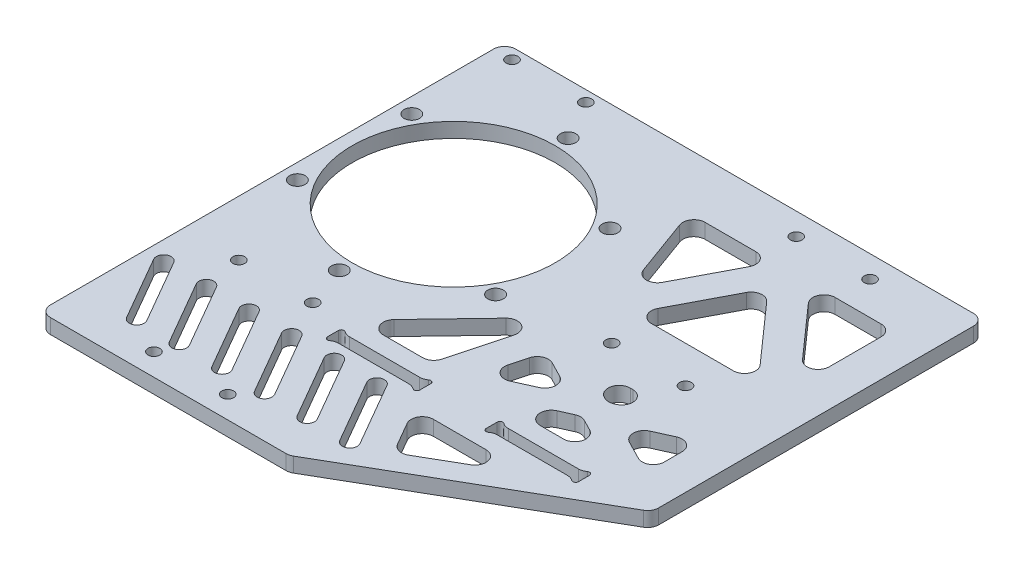
from build123d import *

# Parameters (mm, degrees)
SKETCH_1_W          = 130
SKETCH_1_H          = 90
SKETCH_1_R          = 27.5
SKETCH_1_R_2        = 2.1
SKETCH_1_R_3        = 1.6
EXTRUDE_1_DEPTH     = 4
EXTRUDE_2_DEPTH     = 4
SKETCH_3_R          = 1.6
CUT_EXTRUDE_1_DEPTH = 10
SKETCH_4_R          = 1.6
CUT_EXTRUDE_2_DEPTH = 10
CUT_EXTRUDE_3_DEPTH = 10
FILLET_1_R          = 3
CUT_EXTRUDE_4_DEPTH = 10
FILLET_2_R          = 3


with BuildPart() as part:
    # 草图1 → 凸台-拉伸1 (new body)
    with BuildSketch(Plane(origin=(0, 0, 0), x_dir=(1, 0, 0), z_dir=(0, 1, 0))):
        with Locations((65, 45)):
            Rectangle(SKETCH_1_W, SKETCH_1_H)
        with Locations(Location((31, 45.2, 0), (0, 0, 270))):
            Circle(SKETCH_1_R, mode=Mode.SUBTRACT)
        with Locations(Location((31, 76.2, 0), (0, 0, 270))):
            Circle(SKETCH_1_R_2, mode=Mode.SUBTRACT)
        with Locations(Location((57.846787517, 60.7, 0), (0, 0, 270))):
            Circle(SKETCH_1_R_2, mode=Mode.SUBTRACT)
        with Locations(Location((57.846787517, 29.7, 0), (0, 0, 270))):
            Circle(SKETCH_1_R_2, mode=Mode.SUBTRACT)
        with Locations(Location((31, 14.2, 0), (0, 0, 270))):
            Circle(SKETCH_1_R_2, mode=Mode.SUBTRACT)
        with Locations(Location((4.153212483, 29.7, 0), (0, 0, 270))):
            Circle(SKETCH_1_R_2, mode=Mode.SUBTRACT)
        with Locations(Location((4.153212483, 60.7, 0), (0, 0, 270))):
            Circle(SKETCH_1_R_2, mode=Mode.SUBTRACT)
        with Locations(Location((15, 3, 0), (0, 0, 270))):
            Circle(SKETCH_1_R_3, mode=Mode.SUBTRACT)
        with Locations(Location((35, 3, 0), (0, 0, 270))):
            Circle(SKETCH_1_R_3, mode=Mode.SUBTRACT)
    extrude(amount=EXTRUDE_1_DEPTH)

    # 草图2 → 凸台-拉伸2 (add)
    with BuildSketch(Plane(origin=(0, 4, 0), x_dir=(1, 0, 0), z_dir=(0, 1, 0))):
        Polygon((130, 0), (67.646170928, -36), (0, -36), (0, 0), align=None)
    extrude(amount=-EXTRUDE_2_DEPTH)

    # 草图3 → 切除-拉伸1 (cut)
    with BuildSketch(Plane(origin=(0, 4, 0), x_dir=(1, 0, 0), z_dir=(0, 1, 0))):
        with Locations(Location((25, -30, 0), (0, 0, 270))):
            Circle(SKETCH_3_R)
        with Locations(Location((45, -30, 0), (0, 0, 270))):
            Circle(SKETCH_3_R)
    extrude(amount=-CUT_EXTRUDE_1_DEPTH, mode=Mode.SUBTRACT)

    # 草图4 → 切除-拉伸2 (cut)
    with BuildSketch(Plane(origin=(0, 4, 0), x_dir=(1, 0, 0), z_dir=(0, 1, 0))):
        with Locations(Location((85, 84, 0), (0, 0, 270))):
            Circle(SKETCH_4_R)
        with Locations(Location((105, 84, 0), (0, 0, 270))):
            Circle(SKETCH_4_R)
        with Locations(Location((85, 34, 0), (0, 0, 270))):
            Circle(SKETCH_4_R)
        with Locations(Location((105, 34, 0), (0, 0, 270))):
            Circle(SKETCH_4_R)
        with Locations(Location((5, 87, 0), (0, 0, 270))):
            Circle(SKETCH_4_R)
        with Locations(Location((25, 87, 0), (0, 0, 270))):
            Circle(SKETCH_4_R)
    extrude(amount=-CUT_EXTRUDE_2_DEPTH, mode=Mode.SUBTRACT)

    # 草图2<3> → 切除-拉伸3 (cut)
    with BuildSketch(Plane(origin=(0, 4, 0), x_dir=(1, 0, 0), z_dir=(0, 1, 0))):
        with BuildLine():
            Line((46.5, 0), (45, 0))
            Line((45, 0), (45, -3))
            ThreePointArc((45, -3), (45.75, -3.75), (46.5, -3))
            Line((46.5, -3), (68.5, -3))
            ThreePointArc((68.5, -3), (69.25, -3.75), (70, -3))
            Line((70, -3), (70, 0))
            Line((70, 0), (68.5, 0))
            Line((68.5, 0), (46.5, 0))
        make_face()
        with BuildLine():
            Line((113, -3), (113, 0))
            Line((113, 0), (111.5, 0))
            Line((111.5, 0), (89.5, 0))
            Line((89.5, 0), (88, 0))
            Line((88, 0), (88, -3))
            ThreePointArc((88, -3), (88.75, -3.75), (89.5, -3))
            Line((89.5, -3), (111.5, -3))
            ThreePointArc((111.5, -3), (112.25, -3.75), (113, -3))
        make_face()
        with BuildLine():
            ThreePointArc((46.5, 0), (45.75, 0.75), (45, 0))
            Line((45, 0), (46.5, 0))
        make_face()
        with BuildLine():
            Line((68.5, 0), (70, 0))
            ThreePointArc((70, 0), (69.25, 0.75), (68.5, 0))
        make_face()
        with BuildLine():
            Line((88, 0), (89.5, 0))
            ThreePointArc((89.5, 0), (88.75, 0.75), (88, 0))
        make_face()
        with BuildLine():
            Line((111.5, 0), (113, 0))
            ThreePointArc((113, 0), (112.25, 0.75), (111.5, 0))
        make_face()
    extrude(amount=-CUT_EXTRUDE_3_DEPTH, mode=Mode.SUBTRACT)

    # 圆角1
    fillet_1_edges = [part.edges().sort_by_distance(p)[0] for p in [
        (67.646170928, 2, 36),
        (0, 2, 36),
        (0, 2, -90),
        (130, 2, -90),
        (130, 2, 0),
    ]]
    fillet(fillet_1_edges, radius=FILLET_1_R)

    # 草图5 → 切除-拉伸4 (cut)
    with BuildSketch(Plane(origin=(0, 4, 0), x_dir=(1, 0, 0), z_dir=(0, 1, 0))):
        with BuildLine():
            Line((6.732050808, -6.339745962), (16.732050808, -23.660254038))
            ThreePointArc((16.732050808, -23.660254038), (16, -26.392304845), (13.267949192, -25.660254038))
            Line((13.267949192, -25.660254038), (3.267949192, -8.339745962))
            ThreePointArc((3.267949192, -8.339745962), (4, -5.607695155), (6.732050808, -6.339745962))
        make_face()
        with BuildLine():
            Line((18.279056191, -6.339745962), (28.279056191, -23.660254038))
            ThreePointArc((28.279056191, -23.660254038), (27.547005384, -26.392304845), (24.814954576, -25.660254038))
            Line((24.814954576, -25.660254038), (14.814954576, -8.339745962))
            ThreePointArc((14.814954576, -8.339745962), (15.547005384, -5.607695155), (18.279056191, -6.339745962))
        make_face()
        with BuildLine():
            Line((29.826061575, -6.339745962), (39.826061575, -23.660254038))
            ThreePointArc((39.826061575, -23.660254038), (39.094010768, -26.392304845), (36.36195996, -25.660254038))
            Line((36.36195996, -25.660254038), (26.36195996, -8.339745962))
            ThreePointArc((26.36195996, -8.339745962), (27.094010768, -5.607695155), (29.826061575, -6.339745962))
        make_face()
        with BuildLine():
            Line((41.373066959, -6.339745962), (51.373066959, -23.660254038))
            ThreePointArc((51.373066959, -23.660254038), (50.641016151, -26.392304845), (47.908965344, -25.660254038))
            Line((47.908965344, -25.660254038), (37.908965344, -8.339745962))
            ThreePointArc((37.908965344, -8.339745962), (38.641016151, -5.607695155), (41.373066959, -6.339745962))
        make_face()
        with BuildLine():
            Line((52.920072343, -6.339745962), (62.920072343, -23.660254038))
            ThreePointArc((62.920072343, -23.660254038), (62.188021535, -26.392304845), (59.455970728, -25.660254038))
            Line((59.455970728, -25.660254038), (49.455970728, -8.339745962))
            ThreePointArc((49.455970728, -8.339745962), (50.188021535, -5.607695155), (52.920072343, -6.339745962))
        make_face()
        with BuildLine():
            Line((64.467077727, -6.339745962), (74.467077727, -23.660254038))
            ThreePointArc((74.467077727, -23.660254038), (73.735026919, -26.392304845), (71.002976111, -25.660254038))
            Line((71.002976111, -25.660254038), (61.002976111, -8.339745962))
            ThreePointArc((61.002976111, -8.339745962), (61.735026919, -5.607695155), (64.467077727, -6.339745962))
        make_face()
        Polygon((73.508529611, -8), (81.167295593, -21.265371804), (104.143593539, -8), align=None)
        Polygon((65, 75), (74.430902982, 49.088807011), (87.985735716, 75), align=None)
        Polygon((80.797341547, 44), (114.652939968, 44), (93.356176649, 68.007260469), align=None)
        Polygon((120, 50.027594945), (120, 75), (97.847060032, 75), align=None)
        Polygon((72.888107353, 34), (45.117580773, 5), (65.117580773, 5), align=None)
        Polygon((80.701704351, 5), (113.42265886, 5), (98.11340514, 12.846439281), align=None)
        Polygon((74.402575084, 8.742444076), (78.232515284, 23.035975491), (91.280667048, 16.348416944), align=None)
        Polygon((85.604064397, 26), (112.698085865, 26), (98.280627632, 19.502891419), align=None)
        Polygon((120, 8.371079272), (120, 22.709452649), (105.113365724, 16.000913756), align=None)
    extrude(amount=-CUT_EXTRUDE_4_DEPTH, mode=Mode.SUBTRACT)

    # 圆角2
    fillet_2_edges = [part.edges().sort_by_distance(p)[0] for p in [
        (68.5, 2, 3),
        (46.5, 2, 3),
        (46.5, 2, 0),
        (68.5, 2, 0),
        (111.5, 2, 3),
        (89.5, 2, 3),
        (89.5, 2, 0),
        (111.5, 2, 0),
        (65, 2, -75),
        (87.985735716, 2, -75),
        (74.430902982, 2, -49.088807011),
        (97.847060032, 2, -75),
        (120, 2, -75),
        (120, 2, -50.027594945),
        (73.508529611, 2, 8),
        (104.143593539, 2, 8),
        (81.167295593, 2, 21.265371804),
        (112.698085865, 2, -26),
        (98.280627632, 2, -19.502891419),
        (85.604064397, 2, -26),
        (78.232515284, 2, -23.035975491),
        (91.280667048, 2, -16.348416944),
        (74.402575084, 2, -8.742444076),
        (80.797341547, 2, -44),
        (93.356176649, 2, -68.007260469),
        (114.652939968, 2, -44),
        (72.888107353, 2, -34),
        (65.117580773, 2, -5),
        (45.117580773, 2, -5),
        (120, 2, -8.371079272),
        (105.113365724, 2, -16.000913756),
        (120, 2, -22.709452649),
        (98.11340514, 2, -12.846439281),
        (113.42265886, 2, -5),
        (80.701704351, 2, -5),
    ]]
    fillet(fillet_2_edges, radius=FILLET_2_R)


solid = part.part
